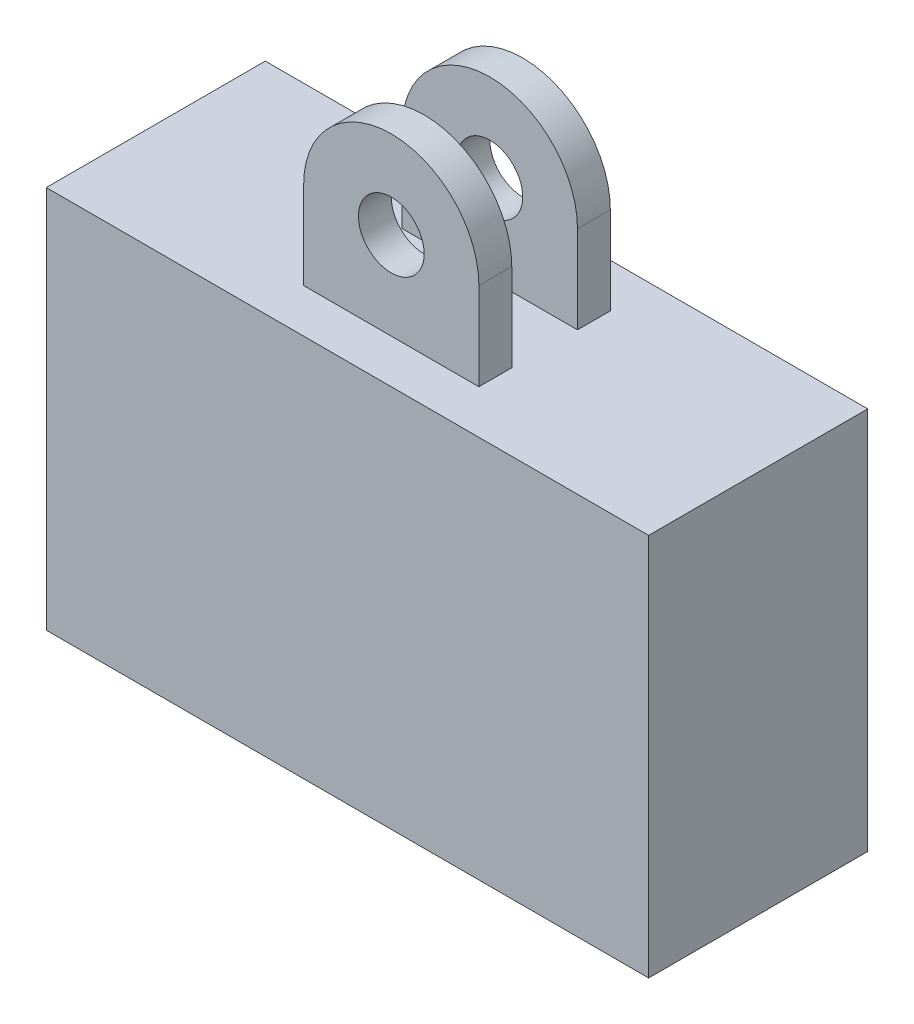
from build123d import *

# Parameters (mm, degrees)
SKETCH1_W               = 55
SKETCH1_H               = 35
BOSS_EXTRUDE1_DEPTH     = 20
SKETCH2_W               = 16
SKETCH2_H               = 12
BOSS_EXTRUDE2_DEPTH     = 16
CUT_EXTRUDE1_DEPTH      = 62.296410988
CUT_EXTRUDE1_DEPTH_BACK = 16
SKETCH3_W               = 16
SKETCH3_H               = 6
SKETCH4_R               = 3
CUT_EXTRUDE2_DEPTH      = 47.200649346


with BuildPart() as part:
    # Sketch1 → Boss-Extrude1 (new body)
    with BuildSketch(Plane.XY):
        Rectangle(SKETCH1_W, SKETCH1_H)
    extrude(amount=BOSS_EXTRUDE1_DEPTH)

    # Sketch2 → Boss-Extrude2 (add)
    with BuildSketch(Plane(origin=(0, 17.5, 0), x_dir=(1, 0, 0), z_dir=(0, 1, 0))):
        with Locations((0, -10)):
            Rectangle(SKETCH2_W, SKETCH2_H)
    extrude(amount=BOSS_EXTRUDE2_DEPTH)

    # Sketch3 → Cut-Extrude1 (cut, two sides: drawn at the far end of the back side and taken through both)
    with BuildSketch(Plane(origin=(0, 33.5, 0), x_dir=(1, 0, 0), z_dir=(0, 1, 0)).offset(-CUT_EXTRUDE1_DEPTH_BACK)):
        with Locations((0, -10)):
            Rectangle(SKETCH3_W, SKETCH3_H)
    extrude(amount=CUT_EXTRUDE1_DEPTH + CUT_EXTRUDE1_DEPTH_BACK, mode=Mode.SUBTRACT)

    # Sketch4 → Cut-Extrude2 (cut, through all)
    with BuildSketch(Plane.XY.offset(16)):
        with Locations((0, 25.5)):
            Circle(SKETCH4_R)
        with BuildLine():
            Line((-8, 25.5), (-21.64466881, 27.690296909))
            Line((-21.64466881, 27.690296909), (-8, 39.036178495))
            Line((-8, 39.036178495), (25.748849804, 31.989915092))
            Line((25.748849804, 31.989915092), (8, 25.5))
            ThreePointArc((8, 25.5), (0, 33.5), (-8, 25.5))
        make_face()
    extrude(amount=-CUT_EXTRUDE2_DEPTH, mode=Mode.SUBTRACT)


solid = part.part
